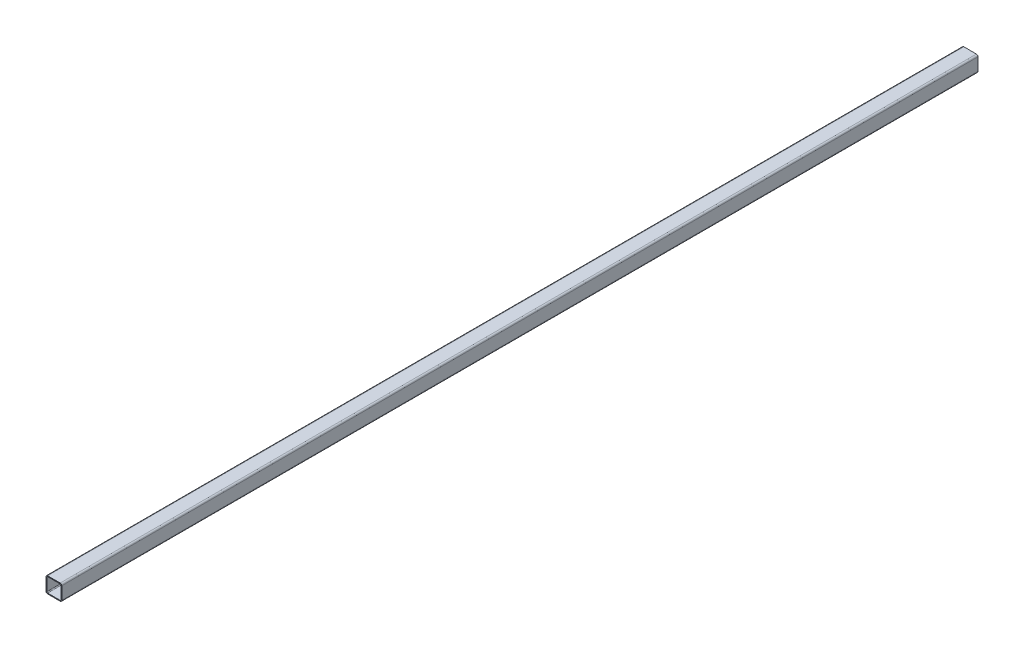
SolidWorks part; units mm, degrees
material "普通碳钢"
ref_plane "Front Plane" through (0, 0, 0) normal (0, 0, 1) x (1, 0, 0)
ref_plane "Top Plane" through (0, 0, 0) normal (0, 1, 0) x (1, 0, 0)
ref_plane "Right Plane" through (0, 0, 0) normal (1, 0, 0) x (0, 0, -1)
sketch "Sketch1" plane through (0, 0, 0) normal (0, 0, 1) x (1, 0, 0)
  line L0 (10, 95) -> (90, 95)
  line L1 (10, 0) -> (90, 0)
  line L2 (0, 10) -> (0, 90)
  line L3 (10, 100) -> (90, 100)
  line L4 (100, 10) -> (100, 90)
  line L5 (95, 10) -> (95, 90)
  line L6 (10, 5) -> (90, 5)
  line L7 (5, 10) -> (5, 90)
  arc A0 (100, 10) -> (90, 0) centre (90, 10) cw
  arc A1 (0, 90) -> (10, 100) centre (10, 90) cw
  arc A2 (100, 90) -> (90, 100) centre (90, 90) ccw
  arc A3 (10, 0) -> (0, 10) centre (10, 10) cw
  arc A4 (95, 90) -> (90, 95) centre (90, 90) ccw
  arc A5 (95, 10) -> (90, 5) centre (90, 10) cw
  arc A6 (10, 5) -> (5, 10) centre (10, 10) cw
  arc A7 (5, 90) -> (10, 95) centre (10, 90) cw
  point P7 (100, 0)
  point P10 (0, 100)
  point P13 (100, 100)
  point P16 (0, 0)
  dimension "D3" = 10
  dimension "D4" = 10
  dimension "D5" = 10
  dimension "D6" = 10
  dimension "D1" = 100
  dimension "D2" = 100
  dimension "D7" = 5
extrude "Boss-Extrude1" add sketch "Sketch1" along normal blind 5800
